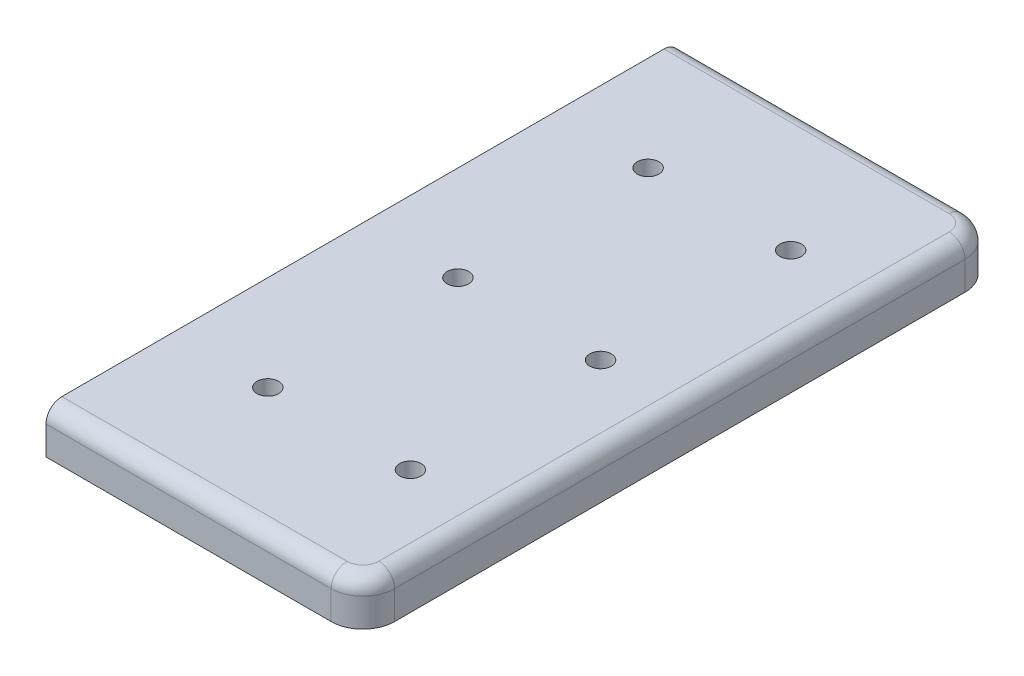
SolidWorks part; units mm, degrees
material "Q235"
ref_plane "Front" through (0, 0, 0) normal (0, 0, 1) x (1, 0, 0)
ref_plane "Top" through (0, 0, 0) normal (0, 1, 0) x (1, 0, 0)
ref_plane "Right" through (0, 0, 0) normal (1, 0, 0) x (0, 0, -1)
sketch "Sketch1" plane through (0, 0, 0) normal (0, 1, 0) x (1, 0, 0)
  line L1 (-50, 100) -> (50, 100)
  line L2 (-50, 100) -> (-50, -100)
  line L3 (-50, -100) -> (50, -100)
  line L4 (50, 100) -> (50, -100)
  line L5 (-50, 100) -> (50, -100) construction
  line L6 (-50, -100) -> (50, 100) construction
  point P0 (0, 0)
  dimension "D1" = 100
  dimension "D2" = 200
extrude "Boss-Extrude1" add sketch "Sketch1" along normal blind 14
chamfer "Chamfer1" [suppressed] distance 15 angle 45
fillet "Fillet1" radius 10 2 edges at (50, 7, -100) (50, 7, 100)
sketch "Sketch2" plane through (0, 14, 0) normal (0, 1, 0) x (1, 0, 0)
  line L0 (27.5, 95) -> (32.5, 95) construction
  line L1 (27.5, 103.25) -> (32.5, 103.25)
  line L2 (27.5, 86.75) -> (32.5, 86.75)
  line L3 (0, 0) -> (28.9214, 0) construction
  line L4 (27.5, -95) -> (32.5, -95) construction
  line L5 (27.5, -103.25) -> (32.5, -103.25)
  line L6 (27.5, -86.75) -> (32.5, -86.75)
  line L7 (50, -90) -> (50, 90) construction
  arc A0 (27.5, 103.25) -> (27.5, 86.75) centre (27.5, 95) ccw
  arc A1 (32.5, 86.75) -> (32.5, 103.25) centre (32.5, 95) ccw
  arc A2 (27.5, -103.25) -> (27.5, -86.75) centre (27.5, -95) cw
  arc A3 (32.5, -86.75) -> (32.5, -103.25) centre (32.5, -95) cw
  point P2 (30, 95)
  point P12 (30, -95)
  dimension "D4" = 190
  dimension "D1" = 16.5
  dimension "D2" = 5
  dimension "D3" = 20
extrude "Cut-Extrude1" [suppressed] cut sketch "Sketch2" against normal through all
sketch "Sketch4" plane through (0, 14, 0) normal (0, 1, 0) x (1, 0, 0)
  line L0 (-27.5, 72.5) -> (-22.5, 72.5) construction
  line L1 (-27.5, 80.75) -> (-22.5, 80.75)
  line L2 (-27.5, 64.25) -> (-22.5, 64.25)
  line L3 (0, 0) -> (50, 0) construction
  line L4 (50, -90) -> (50, 90) construction
  line L5 (-27.5, -72.5) -> (-22.5, -72.5) construction
  line L6 (-27.5, -80.75) -> (-22.5, -80.75)
  line L7 (-27.5, -64.25) -> (-22.5, -64.25)
  arc A0 (-27.5, 80.75) -> (-27.5, 64.25) centre (-27.5, 72.5) ccw
  arc A1 (-22.5, 64.25) -> (-22.5, 80.75) centre (-22.5, 72.5) ccw
  arc A2 (-27.5, -80.75) -> (-27.5, -64.25) centre (-27.5, -72.5) cw
  arc A3 (-22.5, -64.25) -> (-22.5, -80.75) centre (-22.5, -72.5) cw
  point P2 (-25, 72.5)
  point P14 (-25, -72.5)
  dimension "D4" = 145
  dimension "D1" = 16.5
  dimension "D2" = 5
  dimension "D3" = 75
extrude "Cut-Extrude2" [suppressed] cut sketch "Sketch4" against normal through all
sketch "Sketch5" plane through (0, 14, 0) normal (0, 1, 0) x (1, 0, 0)
  line L0 (2.5, 80) -> (7.5, 80) construction
  line L1 (2.5, 88.25) -> (7.5, 88.25)
  line L2 (2.5, 71.75) -> (7.5, 71.75)
  line L3 (0, 0) -> (50, 0) construction
  line L4 (50, -90) -> (50, 90) construction
  line L5 (2.5, -80) -> (7.5, -80) construction
  line L6 (2.5, -88.25) -> (7.5, -88.25)
  line L7 (2.5, -71.75) -> (7.5, -71.75)
  arc A0 (2.5, 88.25) -> (2.5, 71.75) centre (2.5, 80) ccw
  arc A1 (7.5, 71.75) -> (7.5, 88.25) centre (7.5, 80) ccw
  arc A2 (2.5, -88.25) -> (2.5, -71.75) centre (2.5, -80) cw
  arc A3 (7.5, -71.75) -> (7.5, -88.25) centre (7.5, -80) cw
  point P2 (5, 80)
  point P14 (5, -80)
  dimension "D1" = 160
  dimension "D2" = 5
  dimension "D3" = 45
  dimension "D4" = 16.5
extrude "Cut-Extrude3" [suppressed] cut sketch "Sketch5" against normal through all
sketch "Sketch6" plane through (0, 14, 0) normal (0, 1, 0) x (1, 0, 0)
  line L0 (27.5, 57.5) -> (32.5, 57.5) construction
  line L1 (27.5, 65.75) -> (32.5, 65.75)
  line L2 (27.5, 49.25) -> (32.5, 49.25)
  line L3 (50, 0) -> (8.8645, 0) construction
  line L4 (50, -90) -> (50, 90) construction
  line L5 (27.5, -57.5) -> (32.5, -57.5) construction
  line L6 (27.5, -65.75) -> (32.5, -65.75)
  line L7 (27.5, -49.25) -> (32.5, -49.25)
  arc A0 (27.5, 65.75) -> (27.5, 49.25) centre (27.5, 57.5) ccw
  arc A1 (32.5, 49.25) -> (32.5, 65.75) centre (32.5, 57.5) ccw
  arc A2 (27.5, -65.75) -> (27.5, -49.25) centre (27.5, -57.5) cw
  arc A3 (32.5, -49.25) -> (32.5, -65.75) centre (32.5, -57.5) cw
  point P2 (30, 57.5)
  point P14 (30, -57.5)
  dimension "D1" = 115
  dimension "D2" = 16.5
  dimension "D3" = 5
  dimension "D4" = 20
extrude "Cut-Extrude4" [suppressed] cut sketch "Sketch6" against normal through all
fillet "Fillet2" radius 5 5 edges at (-5, 14, 100) (47.0711, 14, 97.0711) (-5, 14, -100) (47.0711, 14, -97.0711) (50, 14, 0)
hole_wizard "M8 Tapped Hole1" positions "Sketch7" profile "Sketch8" tap size "M8" standard "GB"
sketch "Sketch7" plane through (0, 0, 0) normal (0, -1, 0) x (-1, 0, 0)
  line L0 (25, 80) -> (25, 0) construction
  line L1 (25, 0) -> (25, -80) construction
  line L2 (25, -80) -> (-35, -80) construction
  line L3 (-35, -80) -> (-35, 0) construction
  line L4 (-35, 0) -> (-35, 80) construction
  line L5 (-35, 80) -> (25, 80) construction
  line L7 (25, 0) -> (-35, 0) construction
  line L9 (-35, 0) -> (-50, 0) construction
  line L10 (-50, -90) -> (-50, 90) construction
  point P0 (25, 80)
  point P2 (-35, 80)
  point P4 (-35, 0)
  point P6 (25, 0)
  point P8 (25, -80)
  point P10 (-35, -80)
  dimension "D1" = 60
  dimension "D2" = 15
  dimension "D3" = 80
sketch "Sketch8" plane through (-25, 0, -80) normal (1, 0, 0) x (0, 0, -1)
  line L0 (0, 0) -> (0, 14)
  line L1 (0, 14) -> (3.4, 14)
  line L2 (3.4, 14) -> (3.4, 0)
  line L5 (3.4, 0) -> (0, 0)
  line L11 (0, -6.35) -> (0, 107.95) construction
  dimension "通孔螺纹孔钻头直径" = 6.8
  dimension "通孔螺纹孔钻头深度" = 14
cosmetic thread "Hole Thread1" [suppressed] parameters "D2"=8
cosmetic thread "Hole Thread2" [suppressed] parameters "D2"=8
cosmetic thread "Hole Thread3" [suppressed] parameters "D2"=8
cosmetic thread "Hole Thread4" [suppressed] parameters "D2"=8
cosmetic thread "Hole Thread5" [suppressed] parameters "D2"=8
cosmetic thread "Hole Thread6" [suppressed] parameters "D2"=8
sketch "Sketch9" plane through (0, 0, 0) normal (0, -1, 0) x (1, 0, 0)
  line L5 (0, 0) -> (26.6333, 0) construction
  line L6 (-34.9949, 75) -> (35.0051, 75)
  line L7 (-34.9949, 75) -> (-34.9949, 15)
  line L8 (-34.9949, 15) -> (35.0051, 15)
  line L9 (35.0051, 75) -> (35.0051, 15)
  line L10 (35.0051, -75) -> (35.0051, -15)
  line L11 (-34.9949, -15) -> (35.0051, -15)
  line L12 (-34.9949, -75) -> (-34.9949, -15)
  line L13 (-34.9949, -75) -> (35.0051, -75)
  dimension "D1" = 60
  dimension "D2" = 30
  dimension "D3" = 70
extrude "Boss-Extrude2" [suppressed] add sketch "Sketch9" along normal blind 3
sketch "Sketch10" plane through (0, 0, 0) normal (0, -1, 0) x (1, 0, 0)
  line L0 (0, 0) -> (0, 26.7752) construction
  line L1 (-45, 75) -> (-5, 75)
  line L2 (-45, 75) -> (-45, -75)
  line L3 (-45, -75) -> (-5, -75)
  line L4 (-5, 75) -> (-5, -75)
  line L5 (5, 75) -> (5, -75)
  line L6 (45, -75) -> (5, -75)
  line L7 (45, 75) -> (45, -75)
  line L8 (45, 75) -> (5, 75)
  line L9 (-50, -100) -> (-50, 100) construction
  line L10 (-50, 100) -> (40, 100) construction
  line L11 (0, 0) -> (-5, 0) construction
  dimension "D1" = 5
  dimension "D2" = 25
  dimension "D3" = 10
extrude "Boss-Extrude3" add sketch "Sketch10" along normal blind 3
sketch "Sketch11" plane through (0, -3, 0) normal (0, -1, 0) x (1, 0, 0)
  line L0 (-45, -75) -> (-5, -75) construction
  line L1 (-45, 75) -> (-35, 75)
  line L2 (-45, 75) -> (-45, -75)
  line L3 (-45, -75) -> (-35, -75)
  line L4 (-35, 75) -> (-35, -75)
  line L5 (-5, -75) -> (-5, 75) construction
  dimension "D1" = 30
extrude "Cut-Extrude5" cut sketch "Sketch11" against normal blind 3
sketch "Sketch12" plane through (0, -3, 0) normal (0, -1, 0) x (1, 0, 0)
  line L4 (45, 75) -> (5, 75)
  line L5 (5, 75) -> (5, -75)
  line L6 (5, -75) -> (45, -75)
  line L7 (45, -75) -> (45, 75)
  line L8 (45, 75) -> (5, 75)
  line L9 (5, 75) -> (5, -75)
  line L10 (5, -75) -> (45, -75)
  line L11 (45, -75) -> (45, 75)
  line L12 (-35, 75) -> (-35, -75)
  line L13 (-35, -75) -> (-5, -75)
  line L14 (-5, -75) -> (-5, 75)
  line L15 (-5, 75) -> (-35, 75)
  line L16 (-35, 75) -> (-35, -75)
  line L17 (-35, -75) -> (-5, -75)
  line L18 (-5, -75) -> (-5, 75)
  line L19 (-5, 75) -> (-35, 75)
  dimension "D1" = 0
  dimension "D2" = 0
extrude "Cut-Extrude6" cut sketch "Sketch12" against normal blind 10
hole_wizard "M8 Tapped Hole2" positions "Sketch13" profile "Sketch14" tap size "M8" standard "GB"
sketch "Sketch13" plane through (0, 7, 0) normal (0, -1, 0) x (-1, 0, 0)
  line L0 (-5, 0) -> (-25, 0) construction
  line L1 (-5, -75) -> (-5, 75) construction
  line L3 (-25, 75) -> (-25, 60) construction
  line L4 (-5, 75) -> (-45, 75) construction
  point P0 (-25, 60)
  point P2 (-25, 0)
  point P4 (-25, -60)
  dimension "D1" = 120
sketch "Sketch14" plane through (25, 7, -60) normal (1, 0, 0) x (0, 0, -1)
  line L0 (0, 0) -> (0, 21.7929)
  line L1 (0, 21.7929) -> (3.4, 19.75)
  line L2 (3.4, 19.75) -> (3.4, 0)
  line L5 (3.4, 0) -> (0, 0)
  line L10 (0, 21.7929) -> (-3.4, 19.75) construction
  line L11 (0, -6.35) -> (0, 107.95) construction
  dimension "螺纹孔钻头直径" = 6.8
  dimension "螺纹孔钻头深度" = 19.75
  dimension "导头角度" = 118
cosmetic thread "Hole Thread7" parameters "D1"=7, "D2"=8
cosmetic thread "Hole Thread8" parameters "D1"=7, "D2"=8
cosmetic thread "Hole Thread9" parameters "D1"=7, "D2"=8
pattern_linear "LPattern1" count 2 spacing 45 along (-1, 0, 0) of "M8 Tapped Hole2"
fillet "Fillet3" radius 5 8 edges at (45, 3.5, 75) (5, 3.5, 75) (-5, 3.5, 75) (-35, 3.5, 75) (-35, 3.5, -75) (-5, 3.5, -75) (5, 3.5, -75) (45, 3.5, -75)
